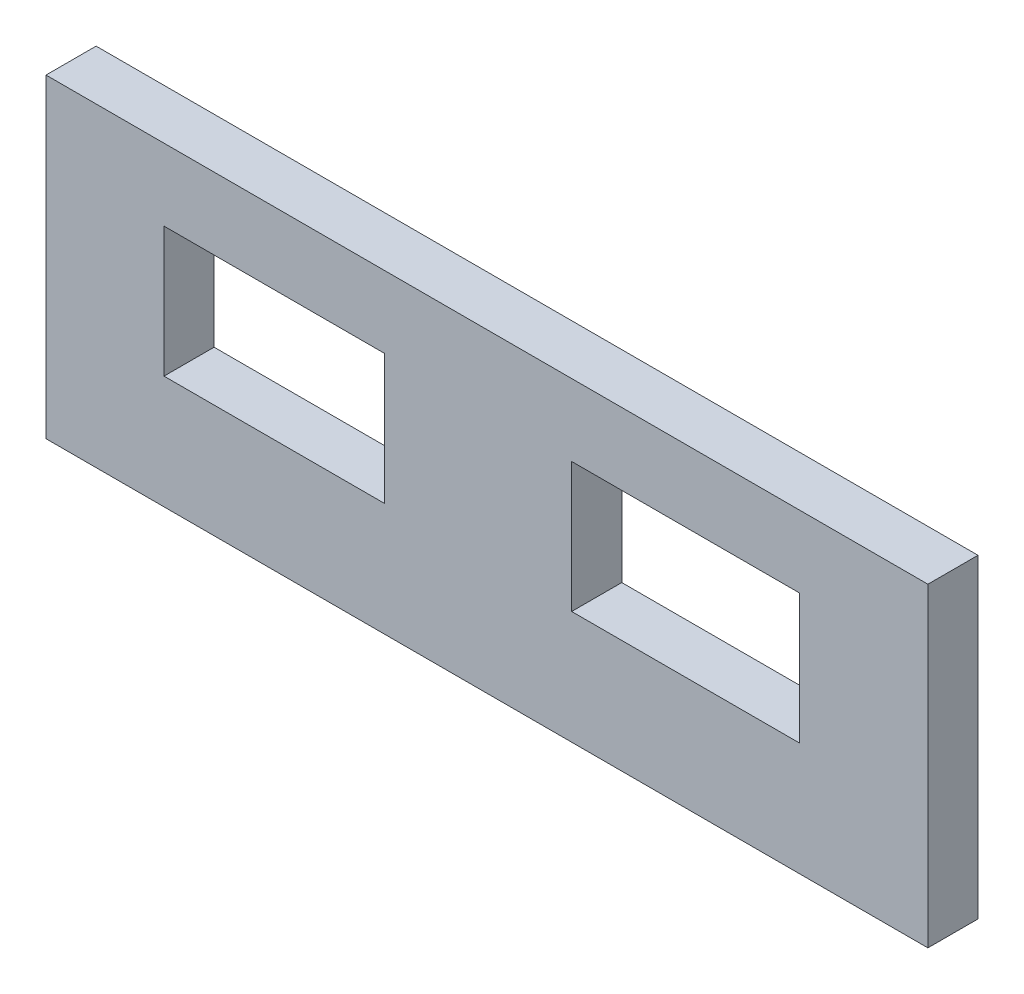
from build123d import *

# Parameters (mm, degrees)
SKETCH1_W           = 616
SKETCH1_H           = 35
BOSS_EXTRUDE1_DEPTH = 220
SKETCH2_W           = 153.942859838
SKETCH2_H           = 90.763998287
SKETCH2_W_2         = 159.281918562
CUT_EXTRUDE1_DEPTH  = 381.117087224


with BuildPart() as part:
    # Sketch1 → Boss-Extrude1 (new body)
    with BuildSketch(Plane(origin=(0, 0, 0), x_dir=(1, 0, 0), z_dir=(0, 1, 0))):
        Rectangle(SKETCH1_W, SKETCH1_H)
    extrude(amount=BOSS_EXTRUDE1_DEPTH)

    # Sketch2 → Cut-Extrude1 (cut, through all)
    with BuildSketch(Plane.XY.offset(17.5)):
        with Locations((-148.603801116, 124.459950708)):
            Rectangle(SKETCH2_W, SKETCH2_H)
        with Locations((138.815526791, 124.459950708)):
            Rectangle(SKETCH2_W_2, SKETCH2_H)
    extrude(amount=-CUT_EXTRUDE1_DEPTH, mode=Mode.SUBTRACT)


solid = part.part
